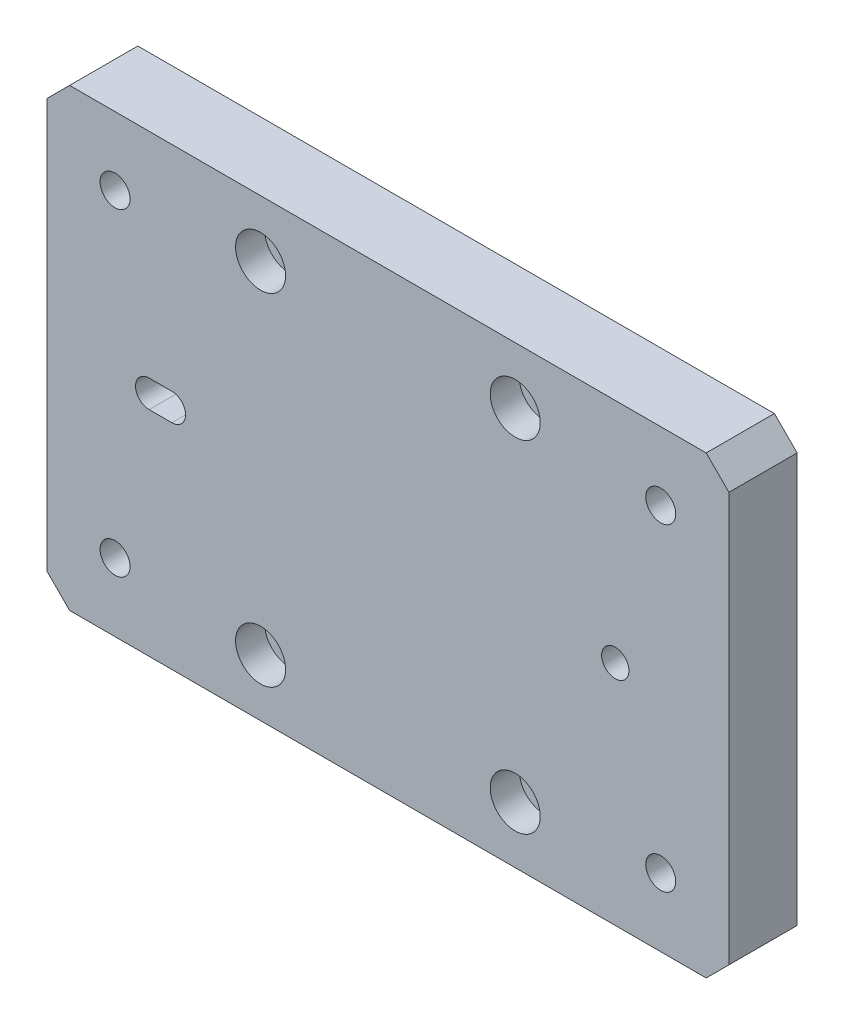
SolidWorks part; units mm, degrees
material "6061"
ref_plane "前视基准面" through (0, 0, 0) normal (0, 0, 1) x (1, 0, 0)
ref_plane "上视基准面" through (0, 0, 0) normal (0, 1, 0) x (1, 0, 0)
ref_plane "右视基准面" through (0, 0, 0) normal (1, 0, 0) x (0, 0, -1)
sketch "草图1" plane through (0, 0, 0) normal (0, 0, 1) x (1, 0, 0)
  line L1 (-75, -50) -> (75, -50)
  line L2 (-75, -50) -> (-75, 50)
  line L3 (-75, 50) -> (75, 50)
  line L4 (75, -50) -> (75, 50)
  line L5 (-75, -50) -> (75, 50) construction
  line L6 (-75, 50) -> (75, -50) construction
  point P0 (0, 0)
  dimension "D1" = 150
  dimension "D2" = 100
extrude "凸台-拉伸1" add sketch "草图1" along normal mid plane 15
hole_wizard "M6 六角凹头螺钉的柱形沉头孔1" positions "草图3" profile "草图2" counterbore size "M6" standard "ISO" end condition through all
sketch "草图3" plane through (0, 0, 7.5) normal (0, 0, 1) x (1, 0, 0)
  line L1 (-28, 37.5) -> (28, 37.5) construction
  line L2 (-28, 37.5) -> (-28, -37.5) construction
  line L3 (-28, -37.5) -> (28, -37.5) construction
  line L4 (28, 37.5) -> (28, -37.5) construction
  line L8 (0, 50) -> (0, -50) construction
  line L9 (75, 50) -> (-75, 50) construction
  line L10 (-75, -50) -> (75, -50) construction
  line L12 (75, 0) -> (-58.1265, 0) construction
  line L13 (75, -50) -> (75, 50) construction
  point P0 (-28, -37.5)
  point P3 (-28, 37.5)
  point P6 (28, 37.5)
  point P9 (28, -37.5)
  dimension "D1" = 75
  dimension "D2" = 56
sketch "草图2" plane through (-28, -37.5, 7.5) normal (1, 0, 0) x (0, -1, 0)
  line L0 (0, 0) -> (0, 15)
  line L1 (0, 15) -> (3.3, 15)
  line L3 (3.3, 15) -> (3.3, 6.4)
  line L4 (3.3, 6.4) -> (5.5, 6.4)
  line L5 (5.5, 6.4) -> (5.5, 0)
  line L7 (5.5, 0) -> (0, 0)
  line L11 (0, -6.35) -> (0, 107.95) construction
  dimension "通孔孔直径" = 6.6
  dimension "通孔孔深度" = 15
  dimension "柱形沉头孔直径" = 11
  dimension "柱形沉头孔深度" = 6.4
chamfer "倒角1" distance 5 angle 45 4 edges at (75, 50, 0) (-75, 50, 0) (-75, -50, 0) (75, -50, 0)
hole_wizard "M6 六角凹头螺钉的柱形沉头孔2" positions "草图4" profile "草图5" counterbore size "M6" standard "ISO" end condition through all
sketch "草图4" plane through (0, 0, -7.5) normal (0, 0, -1) x (-1, 0, 0)
  line L1 (-60, -35) -> (60, -35)
  line L2 (-60, -35) -> (-60, 35)
  line L3 (-60, 35) -> (60, 35)
  line L4 (60, -35) -> (60, 35)
  line L5 (-60, -35) -> (60, 35)
  line L6 (60, 35) -> (60.0049, 34.047)
  point P0 (-60, -35)
  point P2 (-60, 35)
  point P4 (60, 35)
  point P6 (60, -35)
  dimension "D1" = 120
  dimension "D2" = 70
sketch "草图5" plane through (60, -35, -7.5) normal (1, 0, 0) x (0, 1, 0)
  line L0 (0, 0) -> (0, 15)
  line L1 (0, 15) -> (3.3, 15)
  line L3 (3.3, 15) -> (3.3, 8)
  line L4 (3.3, 8) -> (5.5, 8)
  line L5 (5.5, 8) -> (5.5, 0)
  line L7 (5.5, 0) -> (0, 0)
  line L11 (0, -6.35) -> (0, 107.95) construction
  dimension "通孔孔直径" = 6.6
  dimension "通孔孔深度" = 15
  dimension "柱形沉头孔直径" = 11
  dimension "柱形沉头孔深度" = 8
hole_wizard "大小mm 暗销孔1" positions "草图6" profile "草图7" hole size "Ø6.0" standard "ISO" end condition through all
sketch "草图6" plane through (0, 0, -7.5) normal (0, 0, -1) x (-1, 0, 0)
  line L0 (75, 0) -> (-75, 0) construction
  line L1 (75, 45) -> (75, -45) construction
  line L2 (-75, -45) -> (-75, 45) construction
  line L4 (0, 50) -> (0, -58.3622) construction
  line L5 (-70, 50) -> (70, 50) construction
  point P0 (50, 0)
  point P19 (-50, 0)
  dimension "D1" = 100
sketch "草图7" plane through (-50, 0, -7.5) normal (1, 0, 0) x (0, 1, 0)
  line L0 (0, 0) -> (0, 15)
  line L1 (0, 15) -> (3, 15)
  line L2 (3, 15) -> (3, 0)
  line L5 (3, 0) -> (0, 0)
  line L11 (0, -6.35) -> (0, 107.95) construction
  dimension "通孔孔直径" = 6
  dimension "通孔孔深度" = 15
sketch "草图8" plane through (0, 0, -7.5) normal (0, 0, -1) x (-1, 0, 0)
  line L0 (47.5, 0) -> (52.5, 0) construction
  line L1 (47.5, 3) -> (52.5, 3)
  line L2 (47.5, -3) -> (52.5, -3)
  line L3 (-75, 0) -> (77.0762, 0) construction
  line L4 (-75, -45) -> (-75, 45) construction
  arc A0 (47.5, 3) -> (47.5, -3) centre (47.5, 0) ccw
  arc A1 (52.5, -3) -> (52.5, 3) centre (52.5, 0) ccw
  point P2 (50, 0)
  dimension "D2" = 3
  dimension "D1" = 5
extrude "切除-拉伸1" cut sketch "草图8" against normal through all
